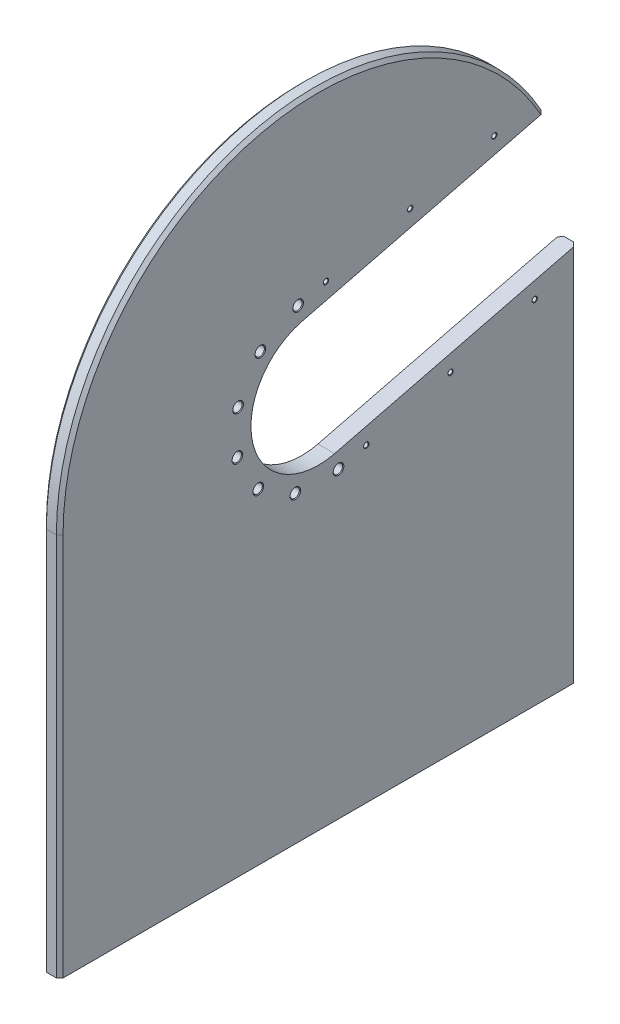
SolidWorks part; units mm, degrees
material "不锈钢板25/304"
ref_plane "Front Plane" through (0, 0, 0) normal (0, 0, 1) x (1, 0, 0)
ref_plane "Top Plane" through (0, 0, 0) normal (0, 1, 0) x (1, 0, 0)
ref_plane "Right Plane" through (0, 0, 0) normal (1, 0, 0) x (0, 0, -1)
sketch "Sketch1" plane through (0, 0, 0) normal (1, 0, 0) x (0, 0, -1)
  line L0 (-387.5, 575) -> (-387.5, 0)
  line L1 (-387.5, 0) -> (387.5, 0)
  line L2 (387.5, 0) -> (387.5, 575)
  line L3 (0, 0) -> (0, 575) construction
  arc A0 (387.5, 575) -> (-387.5, 575) centre (0, 575) ccw
  dimension "D1" = 387.5
  dimension "D2" = 575
  dimension "D3" = 775
extrude "Boss-Extrude1" add sketch "Sketch1" along normal blind 25
sketch "Sketch2" plane through (25, 0, 0) normal (1, 0, 0) x (0, 0, -1)
  line L0 (197.622, 575) -> (0, 575) construction
  line L1 (0, 575) -> (239.3788, 634.6838) construction
  line L2 (-24.4341, 672.9999) -> (338.5593, 763.5043)
  line L3 (24.4341, 477.0001) -> (387.5, 567.5226)
  line L6 (387.5, 575) -> (387.5, 567.5226)
  line L7 (387.5, 0) -> (387.5, 575) construction
  arc A1 (-24.4341, 672.9999) -> (24.4341, 477.0001) centre (0, 575) ccw
  arc A2 (387.5, 575) -> (-387.5, 575) centre (0, 575) ccw construction
  arc A3 (387.5, 575) -> (338.5593, 763.5043) centre (0, 575) ccw
  dimension "D2" = 14
  dimension "D1" = 202
extrude "Cut-Extrude1" cut sketch "Sketch2" against normal up to next
sketch "Sketch3" plane through (25, 0, 0) normal (1, 0, 0) x (0, 0, -1)
  line L0 (-24.4341, 672.9999) -> (-41.665, 742.1093) construction
  line L1 (338.5593, 763.5043) -> (-24.4341, 672.9999) construction
  line L2 (-30.2402, 696.287) -> (333.9386, 787.0869) construction
  circle A0 centre (0, 575) radius 125 construction
  point P8 (-30.2402, 696.287)
  point P11 (11.4825, 706.6896)
  dimension "D1" = 250
  dimension "D2" = 43
hole_wizard "M16 Tapped Hole1" positions "3DSketch1" profile "Sketch4" tap size "M16" standard "GB" end condition through all
sketch3d "3DSketch1"
  point P0 (25, 696.287, 30.2402)
sketch "Sketch4" plane through (25, 696.287, 30.2402) normal (0, 1, 0) x (0, 0, -1)
  line L0 (0, 0) -> (0, 25)
  line L1 (0, 25) -> (7, 25)
  line L2 (7, 25) -> (7, 1.025)
  line L3 (7, 1.025) -> (8.025, 0)
  line L5 (8.025, 0) -> (0, 0)
  line L6 (-7, 1.025) -> (-8.025, 0) construction
  line L11 (0, -6.35) -> (0, 107.95) construction
  dimension "通孔螺纹孔钻头直径" = 14
  dimension "通孔螺纹孔钻头深度" = 25
  dimension "近端锥形沉头孔直径" = 16.05
  dimension "近端锥形沉头孔角度" = 90
cosmetic thread "Hole thread 1" parameters "D2"=16
pattern_circular "CirPattern1" count 12 over 360 about axis through (-0.001, 575, 0) along (1, 0, 0) skipping 1, 2, 3, 4, 5 of "M16 Tapped Hole1"
cosmetic thread "Hole thread 2" parameters "D2"=16
cosmetic thread "Hole thread 3" parameters "D2"=16
cosmetic thread "Hole thread 4" parameters "D2"=16
cosmetic thread "Hole thread 5" parameters "D2"=16
cosmetic thread "Hole thread 6" parameters "D2"=16
cosmetic thread "Hole thread 7" parameters "D2"=16
hole_wizard "M8 Tapped Hole1" positions "3DSketch2" profile "Sketch5" tap size "M8" standard "GB" end condition through all
sketch3d "3DSketch2"
  point P0 (25, 706.6896, -11.4825)
cosmetic thread "Hole thread 8" parameters "D2"=8
sketch "Sketch5" plane through (25, 706.6896, -11.4825) normal (0, 1, 0) x (0, 0, -1)
  line L0 (0, 0) -> (0, 25)
  line L1 (0, 25) -> (3.4, 25)
  line L2 (3.4, 25) -> (3.4, 0.625)
  line L3 (3.4, 0.625) -> (4.025, 0)
  line L5 (4.025, 0) -> (0, 0)
  line L6 (-3.4, 0.625) -> (-4.025, 0) construction
  line L11 (0, -6.35) -> (0, 107.95) construction
  dimension "通孔螺纹孔钻头直径" = 6.8
  dimension "通孔螺纹孔钻头深度" = 25
  dimension "近端锥形沉头孔直径" = 8.05
  dimension "近端锥形沉头孔角度" = 90
pattern_linear "LPattern1" count 3 spacing 130 along (0, 0.2419, -0.9703) of "M8 Tapped Hole1"
cosmetic thread "Hole thread 9" parameters "D2"=8
cosmetic thread "Hole thread 10" parameters "D2"=8
ref_plane "Plane1" through (0, 541.3474, 134.9731) normal (0, 0.9703, 0.2419) x (1, 0, 0)
mirror "Mirror1" about plane through (0, 541.3474, 134.9731) normal (0, 0.9703, 0.2419) of "LPattern1", "M8 Tapped Hole1"
cosmetic thread "Hole thread 11" parameters "D2"=8
cosmetic thread "Hole thread 12" parameters "D2"=8
cosmetic thread "Hole thread 13" parameters "D2"=8
chamfer "Chamfer1" distance 5 6 edges at (25, 287.5, 387.5) (25, 950.0653, 97.3769) (0, 287.5, 387.5) (0, 950.0653, 97.3769) (25, 283.7613, -387.5) (0, 283.7613, -387.5)
